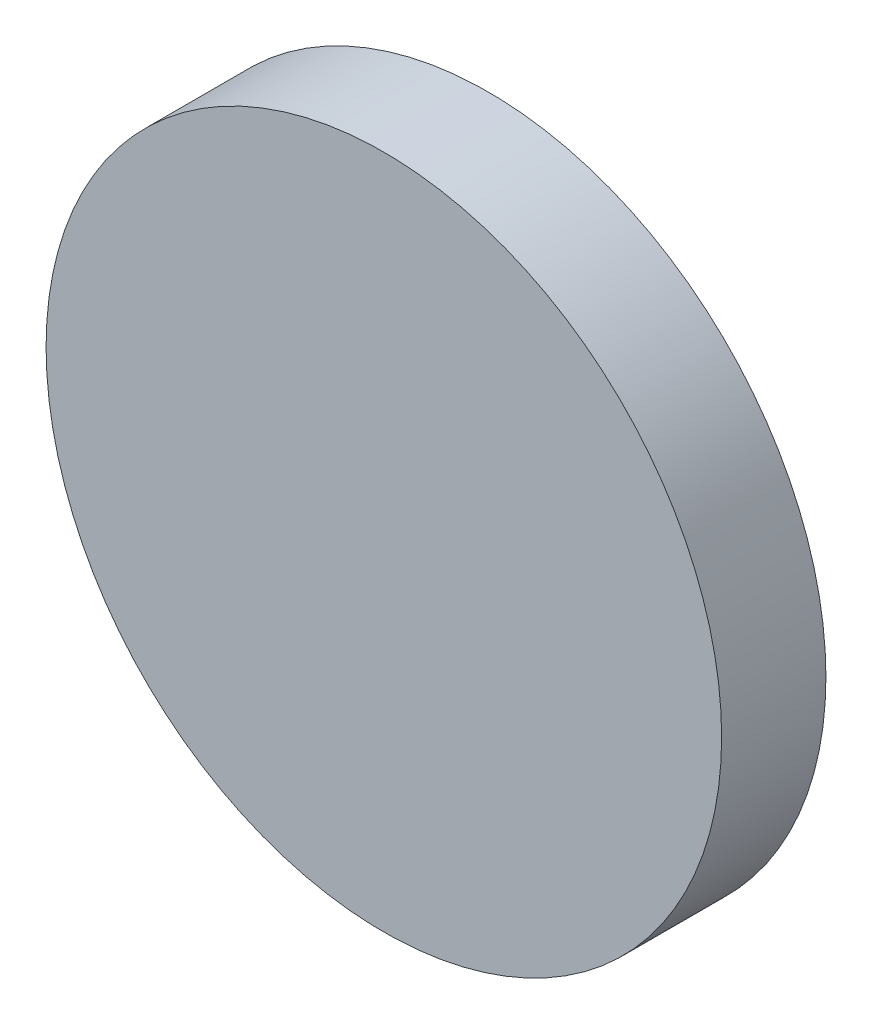
from build123d import *

# Parameters (mm, degrees)
SKETCH2_R           = 74.5
BOSS_EXTRUDE1_DEPTH = 23


with BuildPart() as part:
    # Sketch2 → Boss-Extrude1 (new body)
    with BuildSketch(Plane.XY):
        Circle(SKETCH2_R)
    extrude(amount=BOSS_EXTRUDE1_DEPTH)


solid = part.part
